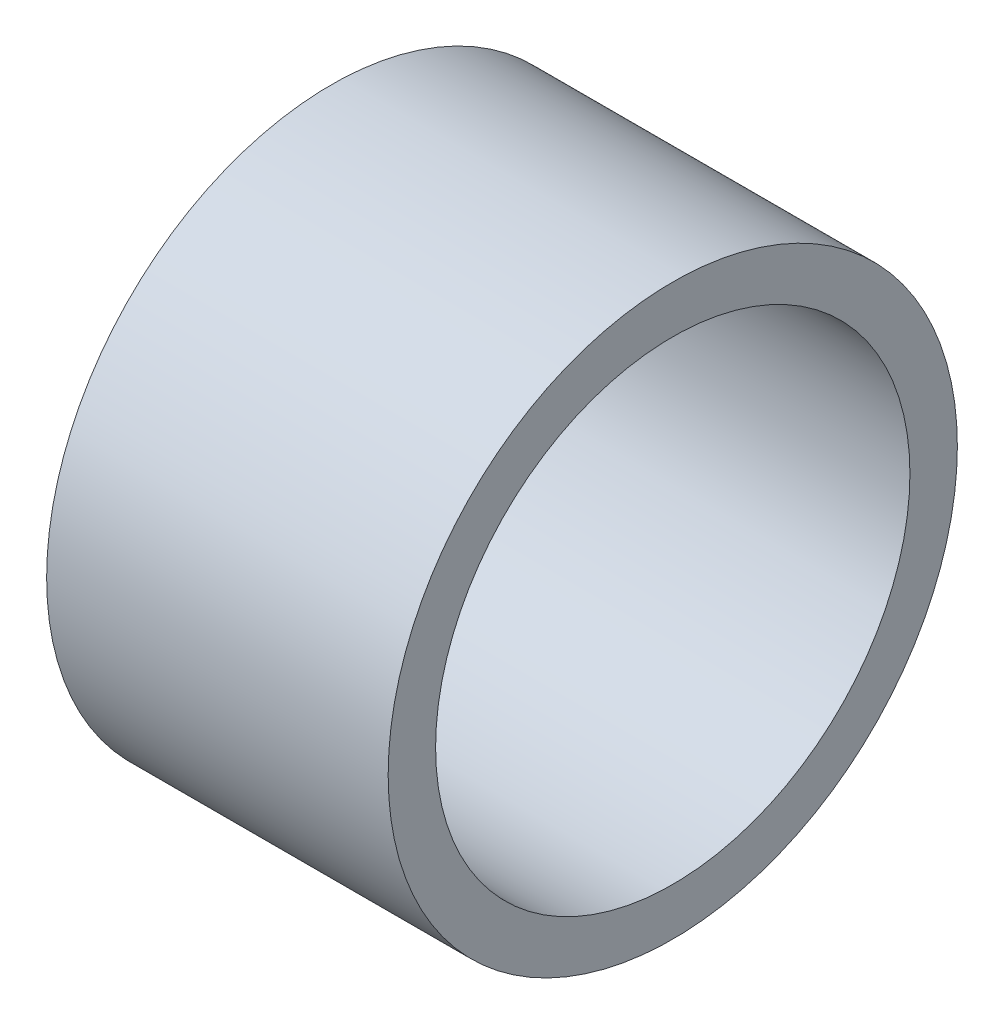
SolidWorks part; units mm, degrees
ref_plane "Front Plane" through (0, 0, 0) normal (0, 0, 1) x (1, 0, 0)
ref_plane "Top Plane" through (0, 0, 0) normal (0, 1, 0) x (1, 0, 0)
ref_plane "Right Plane" through (0, 0, 0) normal (1, 0, 0) x (0, 0, -1)
sketch "Sketch1" plane through (0, 0, 0) normal (0, 0, 1) x (1, 0, 0)
  line L0 (0, 0) -> (49.718, 0) construction
  line L2 (0, 7.5) -> (9, 7.5)
  line L3 (0, 7.5) -> (0, 6.25)
  line L4 (0, 6.25) -> (9, 6.25)
  line L5 (9, 7.5) -> (9, 6.25)
  dimension "D1" = 9
  dimension "D2" = 6.25
  dimension "D3" = 7.5
revolve "Revolve1" add sketch "Sketch1" angle 360 about L0
